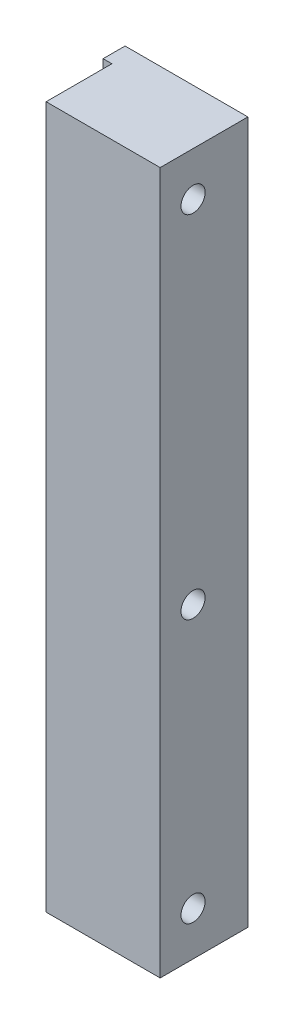
SolidWorks part; units mm, degrees
ref_plane "Front Plane" through (0, 0, 0) normal (0, 0, 1) x (1, 0, 0)
ref_plane "Top Plane" through (0, 0, 0) normal (0, 1, 0) x (1, 0, 0)
ref_plane "Right Plane" through (0, 0, 0) normal (1, 0, 0) x (0, 0, -1)
sketch "Sketch 1" plane through (0, 0, 0) normal (1, 0, 0) x (0, 0, -1)
  line L1 (-10, -80) -> (10, -80)
  line L2 (-10, -80) -> (-10, 80)
  line L3 (-10, 80) -> (10, 80)
  line L4 (10, -80) -> (10, 80)
  line L5 (-10, -80) -> (10, 80) construction
  line L6 (-10, 80) -> (10, -80) construction
  point P0 (0, 0)
  dimension "D1" = 20
  dimension "D2" = 160
extrude "Boss-Extrude 1" add sketch "Sketch 1" along normal blind 28
sketch "Sketch 2" plane through (0, 0, 0) normal (-1, 0, 0) x (0, 0, 1)
  line L0 (10, -80) -> (-10, -80) construction
  line L1 (10, 80) -> (-5, 80)
  line L2 (10, 80) -> (10, -80)
  line L3 (10, -80) -> (-5, -80)
  line L4 (-5, 80) -> (-5, -80)
  dimension "D1" = 15
extrude "Cut-Extrude 1" cut sketch "Sketch 2" against normal blind 2
hole_wizard "M3 Tapped Hole 1" positions "Sketch 4" profile "Sketch 3" tap size "M3" standard "GB"
sketch "Sketch 4" plane through (2, 0, 0) normal (-1, 0, 0) x (0, 0, 1)
  line L0 (-5, -80) -> (10, -80) construction
  line L1 (10, -80) -> (10, 80) construction
  point P0 (2.5, -60)
  dimension "D1" = 20
  dimension "D2" = 7.5
sketch "Sketch 3" plane through (2, -60, 2.5) normal (0, 1, 0) x (0, 0, 1)
  line L0 (0, 0) -> (0, 8.2511)
  line L1 (0, 8.2511) -> (1.25, 7.5)
  line L2 (1.25, 7.5) -> (1.25, 0)
  line L5 (1.25, 0) -> (0, 0)
  line L10 (0, 8.2511) -> (-1.25, 7.5) construction
  line L11 (0, -6.35) -> (0, 107.95) construction
  dimension "螺孔鑽直徑" = 2.5
  dimension "螺孔鑽深度" = 7.5
  dimension "導頭角度" = 118
cosmetic thread "Cosmetic Thread 1" parameters "D1"=6, "D2"=3
pattern_linear "Linear Pattern 1" count 3 spacing 60 along (0, 1, 0) of "M3 Tapped Hole 1"
hole_wizard "M5 Socket Head Cap Screw Counterbore 1" positions "Sketch 6" profile "Sketch 5" counterbore size "M5" standard "JIS" end condition through all
sketch "Sketch 6" plane through (2, 0, 0) normal (-1, 0, 0) x (0, 0, 1)
  line L0 (10, -80) -> (10, 80) construction
  line L1 (-5, -80) -> (10, -80) construction
  point P0 (2.5, -70)
  dimension "D1" = 7.5
  dimension "D2" = 10
sketch "Sketch 5" plane through (2, -70, 2.5) normal (0, 1, 0) x (0, 0, 1)
  line L0 (0, 0) -> (0, 26)
  line L1 (0, 26) -> (2.75, 26)
  line L3 (2.75, 26) -> (2.75, 5)
  line L4 (2.75, 5) -> (5, 5)
  line L5 (5, 5) -> (5, 0)
  line L7 (5, 0) -> (0, 0)
  line L11 (0, -6.35) -> (0, 107.95) construction
  dimension "貫穿孔直徑" = 5.5
  dimension "貫穿孔深度" = 26
  dimension "柱孔直徑" = 10
  dimension "柱孔深度" = 5
pattern_linear "Linear Pattern 2" count 2 spacing 140 along (0, 1, 0) of "M5 Socket Head Cap Screw Counterbore 1"
pattern_linear "Linear Pattern 3" count 2 spacing 60 along (0, 1, 0) of "M5 Socket Head Cap Screw Counterbore 1"
